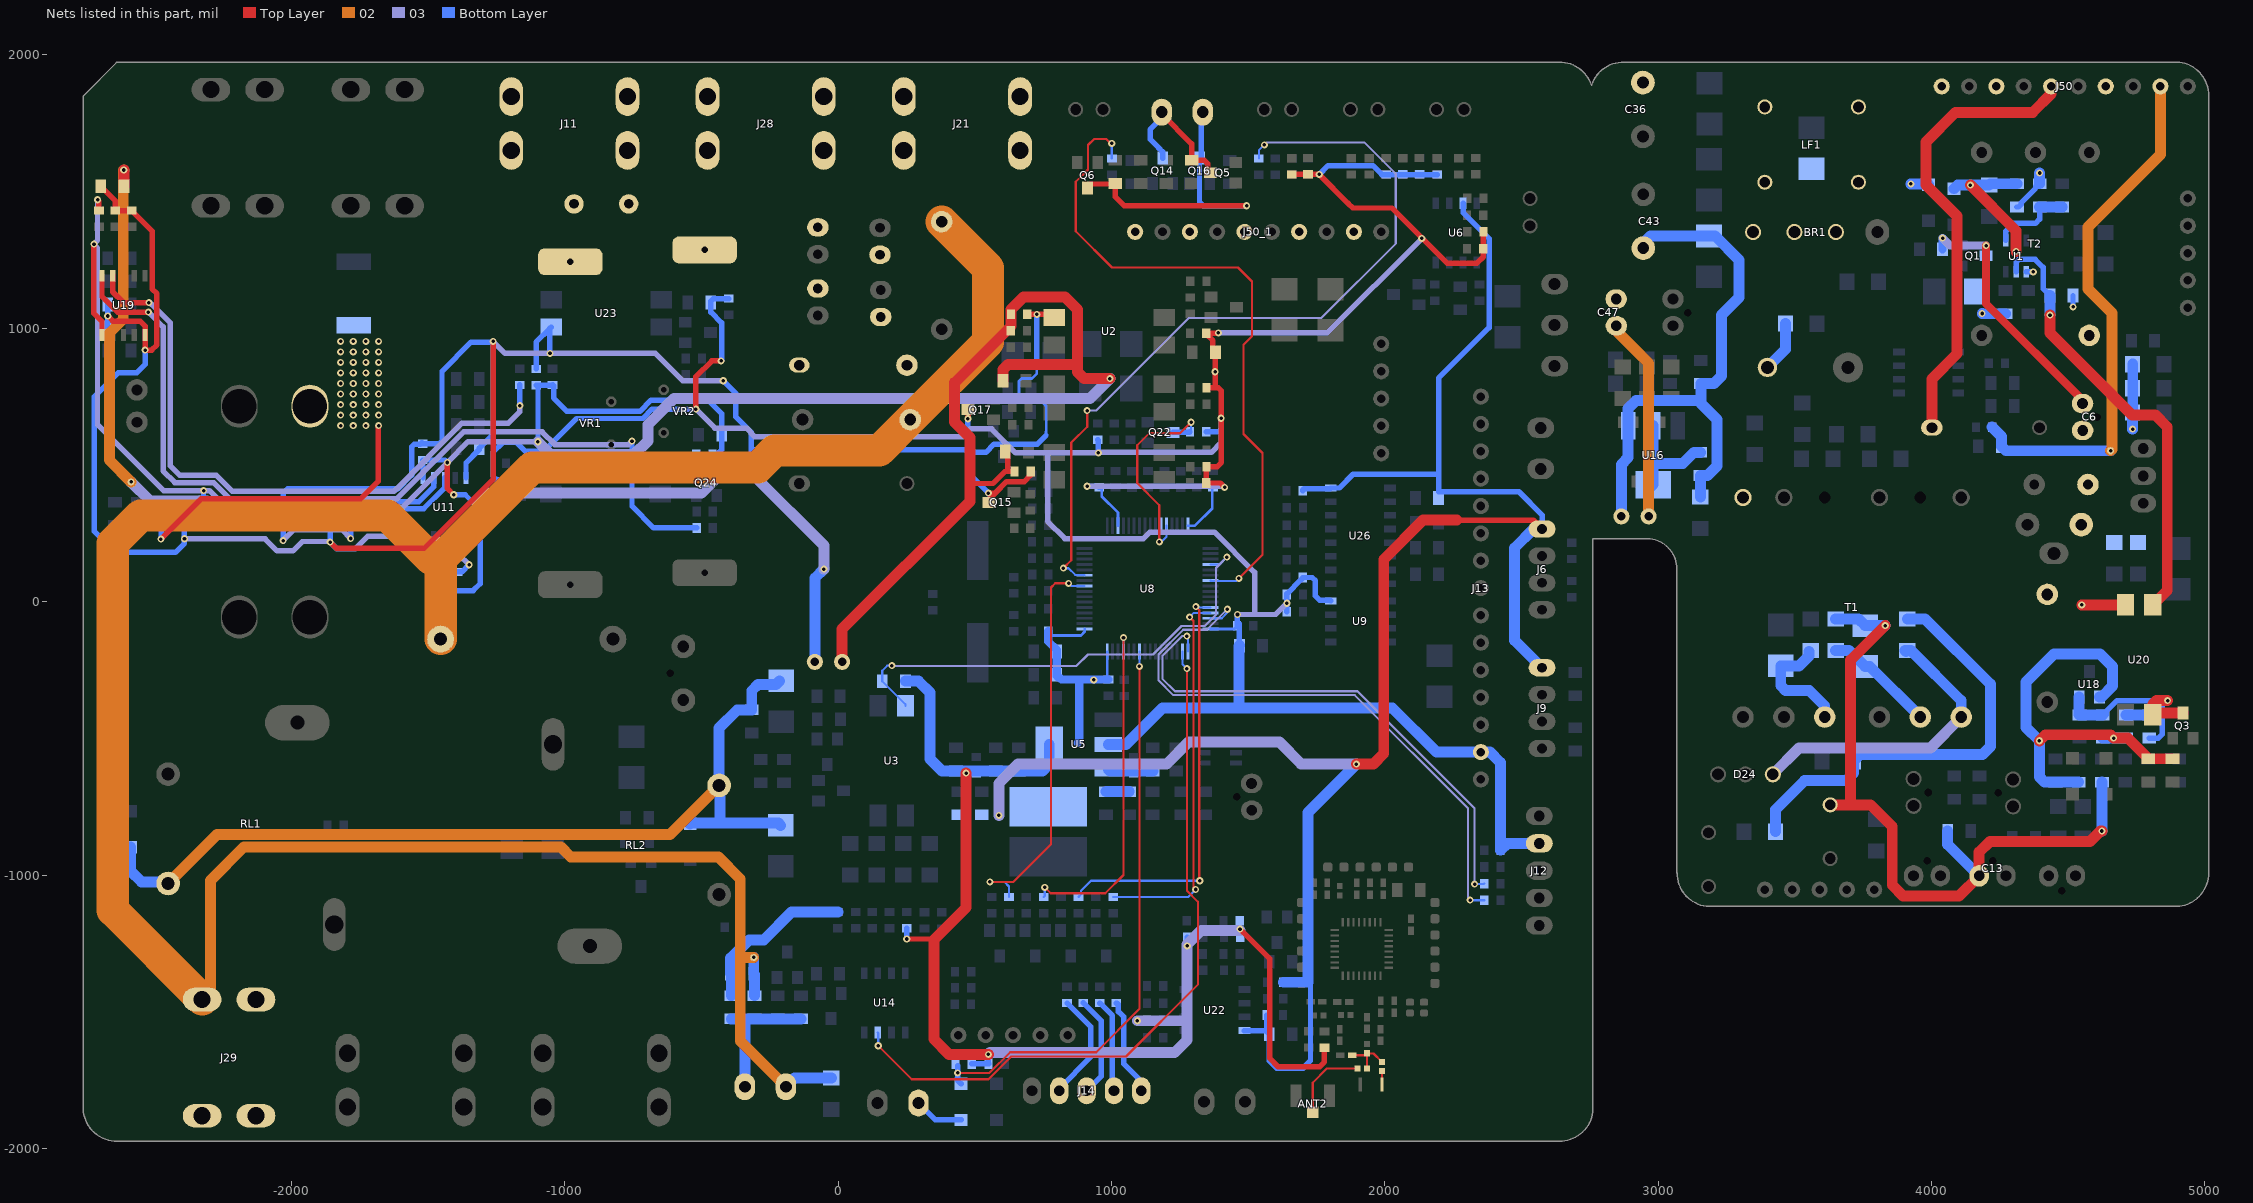
[diagram p0: the nets of this part, all layers, seen from the top]
# Altium PCB MISC105418.PcbDoc (part 4 of 7)
Units mil, origin at the board's own origin, x right, y up, seen from the top; angles counter-clockwise.
Board outline 7774.32 x 3947.04 mil, 4 copper layers (Top Layer, 02, 03, Bottom Layer), stack 30.635 mil thick; 459 components, 285 nets, 1258 pads, 468 vias.
Unrouted connection lines stored in the file: 23.

## Via types
v1: diameter 26, hole 13, Top Layer to Bottom Layer, tented both sides, 468 vias

## Nets (pads, with @x,y where several pads share a name; then routed paths per layer and width w, separated by ;. In a path a pad name is that pad's centre, name@x,y a point inside that pad or via, vN(x,y) a via of type N, cw(c..) or ccw(c..) an arc to the next point about the centre after c; other vN are vias at no path point) (continued)
CHECK-CP: R60.2 R100.2 R103.1 | length 600.5
  Bottom Layer w40: R100.2@-390.91,-1441.5 -390.91,-1363.14 R103.1@-393.23,-1360.82 -392.91,-1360.5 -392.91,-1303.91 -326,-1237 -272,-1237 -169.98,-1134.98 R60.2@-1.11,-1134.98
COIL: C45.1 D12.2 D13.2 D14.2 D15.2 RL1.3 RL2.3 | length 3423.4
  02 w40: RL1.3@-2450.87,-1031 -2271.87,-852 -615.27,-852 RL2.3@-435.21,-671.94
  Bottom Layer w40: D12.2@-2588,-897.94 -2588,-985.39 -2548.57,-1024.82 -2457.06,-1024.82 RL1.3@-2450.87,-1031 ; D13.2@-541.68,-812.74 -539,-810.06 -433.69,-810.06 ; RL2.3@-435.21,-671.94 -435.21,-462.21 -369.05,-396.05 -316.32,-396.05 C45.1@-316,-395.73 -316,-326 -292.57,-302.57 -226.51,-302.57 D14.2@-213.81,-289.87 ; RL2.3@-432.71,-674.45 -432.71,-809.07 -433.69,-810.06 ; D15.2@-210,-818.2 -218.14,-810.06 -433.69,-810.06
CP: C51.1 J26.2 R97.2 R99.1 R100.1 | length 504.5
  Bottom Layer w40: R100.1@-390.91,-1526.14 -338.14,-1526.14 ; J26.2@-341.02,-1774.5 -341.02,-1529.02 -338.14,-1526.14 ; R97.2@-135.91,-1526.14 R99.1@-220.91,-1526.14 C51.1@-305.91,-1526.14 -338.14,-1526.14
CP-ADC-PB1: U8.27
CP-PWM-PA15: U8.50 U14.3 | length 2653.9
  Top Layer w8: v1(147,-1624.43) 269.57,-1747 550,-1747 633,-1664 1053,-1664 1316,-1401 1316,-1098.05 1276,-1058.05 v1(1276,-245)
  Bottom Layer w8: U14.3@145.09,-1575.76 147,-1577.67 v1(147,-1624.43) ; U8.50@1260.05,-182.81 1260.05,-229.05 v1(1276,-245)
D3.3V: C29.1 C31.1 C32.1 C41.2 C54.1 C67.2 C68.2 C69.2 C72.2 C91.2 C95.1 C97.2 C103.1 C104.1 C105.1 C106.1 C107.1 C108.1 C109.2 C115.2 C118.2 FB2.1 J12.4 J13.14 L31.1 R41.1 R53.1 R54.1 R55.1 R63.2 R82.1 R86.2 R107.2 R115.2 R118.2 R133.2 R150.2 R152.2 R154.2 R157.2 R163.2 R173.1 R196.2 R197.1 R233.1 R237.1 R240.1 U5.2 U8.1 U8.19 U8.32 U8.48 U8.64 U9.8 | length 17731.5
  Top Layer w20: v1(-520,704) -520,823 -462,881 v1(-428,881) ; v1(251,-1234) 350,-1234 ; R163.2@1347.83,781.91 1391.09,781.91 1402,771 1402,509 1386.41,493.41 R86.2@1347.83,493.41 1347.24,492.82 1347.24,434.59 C91.2@1346.65,434 1398,434 v1(1414,418) ; 1379.32,781.91 1380.37,782.96 R63.2@1380.37,911.91 1370.69,921.59 1370.69,955.31 1346.65,979.35 C54.1@1346.65,981.91 1389.91,981.91 v1(1391,983) ; v1(1470,-1198) 1579,-1307 1579,-1671 1610,-1702 1761,-1702 1779.09,-1683.91 FB2.1@1779.09,-1632.22 ; R157.2@1659.85,1562.24 1660.23,1562.62 1759.62,1562.62 v1(1760,1563) 1865.88,1457.12 1865.88,1457 1882.88,1440 2026,1440 2228,1238 2337,1238 2359.91,1260.91 C118.2@2359.91,1290.95 2359.91,1352.24 R152.2@2361.09,1353.42
  Top Layer w40: v1(468.5,-627) 468.5,-1119.5 350,-1238 350,-1600 406,-1656 v1(550,-1656)
  03 w20: v1(-520,704) -451,635 -336,635 -305,604 455.63,604 483.63,632 561.56,632 649.56,544 766,544 ; v1(911,422) 1410,422 v1(1414,418) ; v1(1391,983) 1789,983 v1(2135,1329) ; v1(1401,671) 1401,582 1365,546 954,546 v1(952,544) 766,544 ; v1(1461,-47) 1525,-47 ; v1(1641.37,-5.75) 1600.12,-47 1525,-47 ; 766,544 766,293.81 829.24,230.57 1116.57,230.57 1140,254 1376.72,254 1523.36,107.36 1523.36,-45.36 1525,-47
  03 w40: v1(550,-1656) 556,-1650 1230,-1650 1277,-1603 1277,-1534 ; v1(1095,-1533) 1276,-1533 1277,-1534 ; v1@1470,-1203 1328,-1203 1277,-1254 v1(1277,-1259) 1277,-1534
  Bottom Layer w10: C109.2@776.89,-100.13 C109.2@768.53,-108.5 768.53,-121.53 771,-124 888,-124 901.78,-110.22 U8.1@901.78,-100.13 ; C105.1@955,418.28 964.02,409.25 964.02,385.68 1023.83,325.87 U8.19@1023.83,277.82 ; U8.64@984.46,-182.81 984.46,-280.01 C104.1@989,-284.55 ; U8.32@1279.73,277.82 1304.82,277.82 1368.44,341.44 1368.44,418.28 C103.1@1371,418.28 1413.72,418.28 v1(1414,418) ; U8.48@1362.41,-100.13 1449.12,-100.13 C106.1@1467.8,-81.45
  Bottom Layer w19.68: v1(1095,-1533) 1095.35,-1532.65 1129.18,-1532.65 R173.1@1129.53,-1532.29
  Bottom Layer w20: C97.2@-1216.43,386.5 -1215.25,387.69 R133.2@-1215.25,446.23 -1250.28,446.23 -1262,457.94 -1262,547 -1226,583 -1177,583 -1145,551 -1076,551 -957,670 -714,670 -680,704 v1@-521.62,704 ; v1(-428,881) -426,883 -426,1019.77 -465.58,1059.36 R107.2@-465.58,1094.5 -465.58,1099.04 -455.9,1108.72 C95.1@-400,1108.72 ; v1(251,-1234) 251,-1194.87 R82.1@251.44,-1194.43 ; R55.1@489.15,-1690.94 R240.1@550.25,-1690.94 550,-1690.69 v1(550,-1656) ; v1(911,422) 951.28,422 C105.1@955,418.28 ; R41.1@950.04,592.28 952,590.32 v1(952,544) ; v1@1276.63,-1259 R115.2@1276.63,-1227.17 ; R237.1@1346.45,621 1393,621 1401,629 v1(1401,671) ; C106.1@1459.28,-89.98 C106.1@1459.28,-88 1459.28,-48.72 v1(1461,-47) ; C107.1@1467.8,-161 C106.1@1467.8,-81.45 ; R53.1@1641.37,-37.5 v1(1641.37,-5.75) R54.1@1641.37,25.99 1641.37,28.55 1693.4,80.57 1694.48,80.57 1699.64,85.73 C41.2@1699.64,88.29 1734.28,88.29 1746,76.57 1746,21 1762.21,4.79 1799.62,4.79 U9.8@1801.83,2.58 ; v1(1760,1563) 1792,1595 1956,1595 1988.72,1562.28 R154.2@2004.81,1562.28 R150.2@2191.62,1562.28
  Bottom Layer w30: C109.2@768.53,-108.5 768.68,-108.65 768.68,-145.87 C108.1@800,-177.18 ; C108.1@800,-187.28 R197.1@800,-267 800,-272.31 804.68,-277 810,-277 817.55,-284.55 882,-284.55 ; 876,-517 882,-511 882,-284.55 ; C104.1@989,-284.55 882,-284.55
  Bottom Layer w40: R196.2@246.32,-291 294,-291 336,-333 336,-575 380.29,-619.29 L31.1@431.09,-619.29 C31.1@576.09,-619.29 C29.1@661.09,-619.29 747.71,-619.29 772.35,-594.65 U5.2@772.35,-522.5 ; U5.2@988.09,-522.5 1052.5,-522.5 1186,-389 1467,-389 ; C107.1@1467.8,-161 1467,-161.8 1467,-389 ; J12.4@2565.09,-884.3 2448.29,-884.3 R233.1@2423.09,-909.5 2423.09,-589.09 2384.3,-550.3 J13.14@2351.09,-550.3 2188.3,-550.3 2027,-389 1467,-389
  other v1: 935,-286 1379,841
D5V: C17.1 C20.1 C21.1 C22.1 C25.1 C26.1 C28.1 C30.1 C33.1 J6.1 J9.1 L29.2 R36.1 R178.1 U5.3 U6.3 U22.8 U26.16 | length 7729.1
  Top Layer w20: 2263,298 2542.8,298 J6.1@2575.09,265.7
  Top Layer w40: v1(1896,-594) 1958,-594 1996,-556 1996,154.31 2139.69,298 2263,298
  03 w40: v1(588,-782) 588,-664.5 658.5,-594 1202,-594 1282,-514 1614,-514 1694,-594 v1(1896,-594)
  Bottom Layer w20: U22.8@1486.06,-1568.96 1563.48,-1568.96 C21.1@1568.13,-1573.61 ; C22.1@1568.13,-1512.14 C21.1@1568.13,-1573.61 ; C20.1@1699.64,405.7 1699.64,408.26 1704.8,413.42 1799.54,413.42 U26.16@1801.83,415.7 1833.7,415.7 1884,466 2194,466 ; 1728,-1355 1728,-1679 1701,-1706 1604,-1706 1576.65,-1678.65 C21.1@1576.65,-1582.14 C21.1@1568.13,-1573.61 ; U6.3@2286.09,1457.5 2286.09,1422.91 2381,1328 2381,1002.27 2196.32,817.59 2196.32,402 2490,402 2575.09,316.91 J6.1@2575.09,265.7 J6.1@2543.7,265.7
  Bottom Layer w40: C33.1@980.08,-695.17 R36.1@1065.08,-695.17 ; U5.3@988.09,-613.44 993.94,-619.29 C25.1@1151.09,-619.29 ; R178.1@1628.76,-1392.14 1719,-1392.14 1719,-771 v1(1896,-594) ; J6.1@2543.7,265.7 2475,197 2475,-141.57 J9.1@2575.09,-241.66
DB-RX7: R112.2 U19.10 | length 3264.1
  Top Layer w20: U19.10@-2692.74,1192.27 -2692.74,1115.74 -2636,1059 v1(-2523,1059)
  03 w20: v1(-2523,1059) -2469,1005 -2469,478 -2426.23,435.23 -2284.56,435.23 -2225.33,376 -1615.23,376 -1407.23,584 -1370.23,621 -1083.09,621 -1036.09,574 -767,574 v1(-754,587)
  Bottom Layer w20: v1(-754,587) -754,349 -674.5,269.5 R112.2@-517.57,269.5
DB-TX7: R105.2 U19.9 | length 2376.1
  Top Layer w20: U19.9@-2653.37,1192.27 -2653.37,1133.37 -2614,1094 v1(-2521,1094)
  03 w20: v1(-2521,1094) -2519.38,1094 -2513.38,1088 -2510.99,1088 -2443,1020.01 -2443,497 -2408,462 -2274.56,462 -2215.56,403 -1625,403 -1375,653 -1206,653 -1164,695 v1(-1164,717)
  Bottom Layer w20: R105.2@-1164.5,792.75 -1164.25,792.5 -1164.25,717.25 v1(-1164,717)
DBGND: C50.1 C64.2 C74.1 C76.1 C90.1 C92.2 C93.1 C96.1 C98.2 C99.1 C100.2 Q15.3 Q17.3 Q24.3 R96.2 R188.2 R189.1 R190.1 R232.2 R264.1 U2.3 U11.5 U19.5 U23.3 | length 10982.3
  Top Layer w20: R96.2@-2696.85,1519 -2644,1466.15 R190.1@-2644,1430.49 R189.1@-2584,1430.49 -2509,1355.49 -2509,1144 -2492,1127 -2492,939 -2511,920 v1(-2535,920) -2535.13,920.13 -2535.13,975.6 U19.5@-2535.26,975.73 -2535.26,1007.83 -2553.43,1026 -2652.62,1026 v1(-2671.55,1044.93) ; v1(-1858,218) -1836,196 -1513,196 -1262,447 v1(-1262,952) ; v1(475,669) 475.48,669.48 Q17.3@475.48,702.6 ; v1(550,397) 550.22,397.22 574.78,397.22 ; Q15.3@551.37,363 551.37,373.82 574.78,397.22 ; C50.1@692.07,1050.81 v1(727,1050.81) 779.31,1050.81 U2.3@791.21,1038.91 ; C90.1@704.52,476 704.52,462.52 681,439 616.56,439 574.78,397.22
  03 w20: v1(-2391,230) -2096,230 -2052,186 -1994,186 -1960,220 -1860,220 v1(-1858,218) -1834.31,194.31 -1766,194.31 -1721.31,239 -1587,239 -1519,171 -1386,171 v1(-1350,135) ; v1(-1262,952) -1218,908 v1(-1054,908) -668,908 -568,808 v1(-420,808)
  Bottom Layer w10: 727,872 727,834 709,816 671,816 662,807 662,748 675,735 742.56,735 761,716.56 761,622.06 760.49,621.55 760.49,608
  Bottom Layer w20: C100.2@-2671.55,1002.7 v1(-2671.55,1044.93) R188.2@-2671.55,1087.17 ; C99.1@-2561.45,278.77 C99.1@-2560.91,279.31 -2521.22,319 -2431.86,319 C98.2@-2392.18,279.31 ; v1(-2535,920) -2535,868 -2565,838 -2633,838 -2721,750 -2721,257 -2644,180 -2424,180 -2391,213 v1(-2391,230) -2391.59,230.59 -2391.59,278.72 C98.2@-2392.18,279.31 ; C92.2@-2321.4,313.04 -2323.96,313.04 -2348,289 -2382.49,289 C98.2@-2392.18,279.31 ; C76.1@-2030.15,363.96 -2030.15,395.85 -2013,413 -1610,413 -1560,463 -1560,566.33 -1550.33,576 -1528.72,576 -1523,581.72 C64.2@-1519,577.72 -1458.28,577.72 -1449,587 -1449,842.5 -1342.5,949 -1265,949 v1(-1262,952) -1262,611.98 R232.2@-1312.47,561.5 ; C74.1@-1861.91,279.31 -1858,275.41 v1(-1858,218) ; R264.1@-1391.91,108.78 -1376.22,108.78 v1(-1350,135) ; U11.5@-1361.17,452.77 -1361.17,507.5 R232.2@-1312.74,555.93 ; C93.1@-1104.5,851.02 -1104.5,949.31 U23.3@-1054,999.81 ; v1(-1054,908) U23.3@-1054,999.81 ; U23.3@-1049.31,1004.5 U23.3@-1054,999.81 ; C96.1@-518.75,539.5 -518.75,496.75 -502.76,480.76 Q24.3@-481.68,480.76 -339.24,480.76 -317,503 -317,556 ; v1(-420,808) -375,763 -375,677 -317,619 -317,556 ; 475,547 v1(475,669) ; 475,556 -317,556 ; v1(550,397) 475,472 475,546 541,546 571,576 728.49,576 760.49,608 ; 727,872 v1(727,1050.81) ; R232.2@-1312.74,555.93 -1312.47,556.19 R232.2@-1312.47,561.5 ; R232.2@-1312.74,555.93 -1312.74,561.24 R232.2@-1312.47,561.5
EARTH: C51.2 C120.1 FB1.2 J21.1 J26.1 J29.1 J50.9 J50_1.9 R103.2 R192.1 Y2.2 Y3.1 ZC1.1 | length 11901
  02 w40: J29.1@-2326.43,-1455.4 -2296,-1424.98 -2296,-1020 -2174,-898 -1014,-898 -978,-934 -438,-934 -358,-1014 -358,-1301.42 ; v1(-308.58,-1301.42) -358,-1301.42 ; J26.1@-191.02,-1774.5 -358,-1607.52 -358,-1301.42 ; v1(4655,552) 4660,557 4660,1056 4571.94,1144.06 4571.94,1369.94 4837,1635 J50.9@4837,1885
  02 w118.11: J29.1@-2326.43,-1455.4 -2653,-1128.83 -2653,214 -2552,315 -1648,315 -1489.04,156.04 -1453.96,156.04 ; ZC1.1@-1453.96,-137 -1453.96,156.04 ; Y2.2@379,1389.85 548,1220.85 548,950.15 Y3.1@263.85,666 150.85,553 -232,553 -294,491 -1119,491 -1453.96,156.04
  Bottom Layer w40: v1(-308.58,-1301.42) R103.2@-308.58,-1360.82 -305.91,-1363.5 C51.2@-305.91,-1441.5 ; J26.1@-191.02,-1774.5 -159.46,-1742.94 FB1.2@-24.91,-1742.94 ; C120.1@4221.5,638.5 4255.22,604.78 R192.1@4255.22,568.5 4271.72,552 v1(4655,552)
EL3.3V: 2*2.54.1 ?.1 C47.1 C49.2 C50.2 C64.1 C90.2 C92.1 C93.2 C96.2 R61.2 R66.1 R89.1 R104.2 R110.1 R147.2 R162.2 U11.1 U16.2 U19.1 | length 11471.1
  Top Layer w19.68: v1(-2722,1308) -2723,1307 -2723,1055.59 -2692.74,1025.33 U19.1@-2692.74,975.73 ; v1(-2709,1470) -2704,1465 R147.2@-2704,1430.49 ; v1(-1429.38,509) -1429.38,414.38 v1(-1406,391) ; 495,432 566,432 610,476 C90.2@645.07,476 ; R66.1@611.35,549 620.53,539.82 620.53,483.87
  Top Layer w40: 2*2.54.1@14.72,-220.24 14.72,-100.28 482,367 482,601 425.86,657.14 425.86,800.86 632.62,1007.62 C50.2@632.62,1050.81 632.62,1068.93 678,1114.31 829.69,1114.31 875,1069 875,876 ; R89.1@602.74,808.3 602.74,849.74 621,868 867,868 875,876 ; v1(994,816) 899,816 875,840 875,876
  02 w40: C47.1@2828.59,1008.98 2965,872.57 ?.1@2965,312
  03 w19.68: v1(-2709,1470) -2709,1321 v1(-2722,1308) -2722,1306.31 -2709,1293.31 -2709,648 -2467.23,406.23 v1(-2321,406.23) -2300.23,406.23 -2240,346 -1592.38,346 v1(-1429.38,509) -1353.38,585 v1(-1098,585)
  03 w40: v1(-1098,585) -1051,538 -746,538 -696,588 -696,647 -600,743 921,743 v1(994,816)
  Bottom Layer w19.68: C92.1@-2321.4,372.48 -2321.2,372.69 -2321.2,406.03 v1(-2321,406.23) ; U11.1@-1518.65,452.77 -1518.65,517.92 C64.1@-1519,518.28 -1438.65,518.28 v1(-1429.38,509) ; R162.2@-1452.52,109.39 R162.2@-1451.91,108.78 -1451.91,62.27 -1429.64,40 -1335,40 -1309,66 -1309,336 -1364,391 v1(-1406,391) ; C93.2@-1104.5,791.57 -1103.32,791.57 -1098,786.26 v1(-1098,585)
  Bottom Layer w20: C93.2@-1103.32,791.57 -1045.69,791.57 R104.2@-1044.5,792.75 -1040.98,789.23 -1040.98,744.98 -992,696 -724.77,696 -683.77,737 -476,737 -425.58,686.58 R110.1@-425.58,610.76 -425.58,556.42 -442.5,539.5 C96.2@-459.3,539.5
  Bottom Layer w40: ?.1@2965,312 2965,412.29 U16.2@2981,428.29 2981,503 ; U16.2@2981,644.04 2981,505 3089.65,505 3130.98,546.32 C49.2@3154,546.32
Emer-DI-PB2: Q22.3 R237.2 U8.28 | length 792.7
  Top Layer w8: v1(1175,218.65) 1175,353 1094,434 1094,572.02 1137.98,616 1250.73,616 v1(1291,656.27)
  Bottom Layer w8: v1(1175,218.65) 1182.65,218.65 1200.99,236.99 U8.28@1200.99,277.82 ; R237.2@1287,621 1291,625 v1(1291,656.27)
  Bottom Layer w20: Q22.3@1225.26,619 1285,619 R237.2@1287,621
GND: BR1.4 C1.2 C2.2 C3.2 C5.2 C6.2 C62.2 CY1.2 R7.2 R13.2 R16.2 R241.2 T1.6 U1.1 U20.4 ZD1.1 | length 969.4
  Top Layer w39.37: v1(4549,-12) 4708.8,-12 U20.4@4709.09,-11.71
  Bottom Layer w19.68: C3.2@4312.09,1443.7 4317.41,1443.7 4327.25,1453.54 4327.25,1458.86 4379.94,1511.54 4379.94,1518.5 4389.78,1528.35 C2.2@4395,1528.35 ; U1.1@4346.4,1206.52 v1(4371.61,1206.52) ; v1(4517.32,1078) C1.2@4517.32,1120
  Bottom Layer w39.37: C62.2@3399.36,857 3465.44,923.08 C5.2@3465.44,1017 ; v1(3924,1528) 3986.49,1528 ZD1.1@3989.09,1525.39 ; v1(4185,1054) 4185.84,1053.16 R7.2@4270.09,1053.16 ; C2.2@4395,1528.35 v1(4395,1568) ; v1(4735,631) 4735,691.56 R241.2@4735.44,692 R13.2@4735.44,780.5 R16.2@4735.44,869
IN: C76.2 R145.1 U11.3 | length 928.3
  03 w20: v1(-2030,223) -1989.91,263.09 -1815.09,263.09 v1(-1783,231)
  Bottom Layer w19.68: v1(-1783,231) -1783,305.67 -1780.33,308.33 -1783,311 -1754.16,339.84 -1516.16,339.84 -1439.91,416.09 U11.3@-1439.91,452.77
  Bottom Layer w20: R145.1@-2119.69,279.31 C76.2@-2030.15,279.31 -2030.15,223.15 v1(-2030,223)
IP: C74.2 R123.1 U11.2 | length 523
  Bottom Layer w20: R123.1@-1946.14,363.96 C74.2@-1861.92,364.96 ; C74.2@-1861.91,363.96 -1860.18,365.69 -1533.32,365.69 -1479.28,419.72 U11.2@-1479.28,452.77
IP2: pad.1@-1932,715 R182.1 R183.2 | length 1136.7
  Top Layer w20: v1(-2477,229) -2329,377 -1746,377 -1682.15,440.85 -1682.15,642.85 v1(-1681,644)
  Bottom Layer w20: v1(-2477,229) -2476.66,229.34 R182.1@-2476.66,279.31
  other v1: -1820,644 -1773.67,644 -1727.33,644 -1820,682.5 -1773.67,682.5 -1727.33,682.5 -1681,682.5 -1820,721 -1773.67,721 -1727.33,721 -1681,721 -1820,759.5 -1773.67,759.5 -1727.33,759.5 -1681,759.5 -1820,798 -1773.67,798 -1727.33,798 -1681,798 -1820,836.5 -1773.67,836.5 -1727.33,836.5 -1681,836.5 -1820,875 -1773.67,875 -1727.33,875 -1681,875 -1820,913.5 -1773.67,913.5 -1727.33,913.5 -1681,913.5 -1820,952 -1773.67,952 -1727.33,952 -1681,952
JTAG_TCK: R235.2 U8.49 | length 1913.2
  03 w8: v1(1276,-126) 1258.8,-126 1186.13,-198.67 1186.13,-282.13 1232,-328 1900,-328 2328,-756 v1(2328,-1033)
  Bottom Layer w8: v1(1276,-126) 1279.73,-129.73 U8.49@1279.73,-182.81 ; v1(2328,-1033) 2362.14,-1033 R235.2@2363.65,-1031.5
JTAG_TMS: R234.2 U8.46 | length 2214.6
  03 w8: v1(1424,-28) 1349,-103 1262,-103 1172,-193 1172,-288 1226,-342 1890,-342 2304,-756 2304,-1084 v1(2312,-1092)
  Bottom Layer w8: U8.46@1362.41,-60.76 1403.24,-60.76 1424,-40 v1(1424,-28) ; v1(2312,-1092) 2312.5,-1092.5 R234.2@2363.65,-1092.5
L1: BR1.3 D11.1 LF1.1
L2: F1.1 J11.1
L-3: CX2.1 J50.1 J50_1.1 L27.2 LF1.2
L-PLC: CX3.2 F1.2 J50.5 J50_1.5 L26.1 VR1.2 | length 1687.9
  Top Layer w40: CX3.2@4001.09,636.5 4001.09,815.09 4093,907 4093,1411 3980,1524 3980,1682 4088,1790 4370,1790 4437,1857 J50.5@4437,1885
LED-4: J14.5 R126.1 | length 360.6
  Bottom Layer w20: R126.1@1017.25,-1468.34 1019.81,-1468.34 1024.97,-1473.5 1024.97,-1499.29 1044,-1518.32 1044,-1690 1108.98,-1754.98 J14.5@1108.98,-1789.5
LED-Breath: J14.4 R214.1 | length 342.6
  Bottom Layer w20: R214.1@957.25,-1468.34 1003,-1514.09 1003,-1757.05 1008.98,-1763.02 J14.4@1008.98,-1789.5
LED-Breath2-PA12: R127.2 U8.45 | length 1401.9
  Top Layer w8: v1(1286,-56.68) 1300,-70.68 1300,-1045 v1(1308,-1053)
  Bottom Layer w8: R127.2@1005.98,-1080.05 1280.95,-1080.05 v1(1308,-1053) ; v1(1286,-56.68) 1286,-56.08 1301,-41.08 U8.45@1362.41,-41.08
LED-Breath-PA11: R48.2 U8.44 | length 1539.8
  Top Layer w8: v1(1309,-18.08) 1309,-19.39 1321.07,-31.46 1321.07,-528.91 1321,-528.98 1321,-1019.15 v1(1323,-1021.15)
  Bottom Layer w8: R48.2@879.04,-1080.05 888.42,-1070.66 888.42,-1057.58 925,-1021 1322.85,-1021 v1(1323,-1021.15) ; v1(1309,-18.08) 1312.32,-21.39 U8.44@1362.41,-21.39
LED-EREE: J14.3 R213.1 | length 370.2
  Bottom Layer w20: R213.1@897.25,-1468.07 962,-1532.82 962,-1736.47 J14.3@908.98,-1789.5
LED-EREE-PB8: R47.2 U8.61 | length 1281.2
  Top Layer w8: v1(756,-1045) 778,-1067 977,-1067 1044,-1000 v1(1044,-131.69)
  Bottom Layer w8: R47.2@752.1,-1080.05 756,-1076.15 v1(756,-1045) ; U8.61@1043.51,-182.81 1043.76,-182.57 1043.76,-131.93 v1(1044,-131.69)
LED-RUN: J14.2 R125.1 | length 404.6
  Bottom Layer w20: J14.2@808.98,-1789.5 808.98,-1780.02 924,-1665 924,-1554.89 R125.1@837.45,-1468.34
LED-RUN-PC1: R51.2 U8.9 | length 1468.6
  Top Layer w8: v1(555,-1025) 641.52,-1025 779,-887.52 779,52 794,67 v1(843,67)
  Bottom Layer w8: v1(555,-1025) 608,-1025 625.16,-1042.16 R51.2@625.16,-1080.05 ; v1(843,67) 852.65,57.35 U8.9@901.78,57.35
M+: J15.1 Q5.3 Q14.3 R136.1 | length 528.2
  Top Layer w20: J15.1@1184.09,1790.5 1184.09,1783.91 1293.26,1674.74 R136.1@1293.26,1614.34 1339.66,1614.34 1351.37,1602.63 1351.37,1578.69 1361.06,1569 Q5.3@1362,1569
  Bottom Layer w20: J15.1@1184.09,1790.5 1184.09,1769.56 1141,1726.47 1141,1692 1173,1660 1173,1658.99 1187.09,1644.89 Q14.3@1187.09,1622.14
M-: J15.2 Q6.3 Q16.3 R130.1 | length 1164.3
  Top Layer w19.68: Q6.3@912.26,1513.82 912.26,1517.76 922.1,1527.6 1012.18,1527.6 R130.1@1014.26,1529.68 1014.26,1480.74 1047,1448 v1(1494,1448)
  Bottom Layer w19.68: Q16.3@1322.09,1622.14 1322.09,1461.91 1336,1448 v1(1494,1448)
  Bottom Layer w20: Q16.3@1322.09,1622.14 1328.09,1628.14 1328.09,1784.5 J15.2@1334.09,1790.5
M-N-DRV-PC8: R57.2 U8.39 | length 2484.8
  Top Layer w8: v1(1001,1676) 997.64,1676 981.64,1692 935.81,1692 914,1670.19 914,1581 869.09,1536.09 869.09,1354.91 1001.84,1222.16 1462.84,1222.16 1514,1171 1514,971 1483,940 1483,613 1552.44,543.56 1552.44,171.44 v1(1466,85)
  Bottom Layer w8: v1(1001,1676) 1001,1621.78 R57.2@1002.09,1620.69 ; U8.39@1362.41,77.03 1363.72,75.72 1456.72,75.72 v1(1466,85)
M/ScR-DRV-PC3: R56.1 U8.11 | length 2928
  Top Layer w8: v1(824.18,122.82) 853,151.64 853,582 911,640 v1(911,699)
  03 w8: v1(911,699) 944.67,699 1283.67,1038 1768.4,1038 2040,1309.6 2040,1565 1926,1679 1567,1679 v1(1559,1671)
  Bottom Layer w8: v1(824.18,122.82) 824.86,122.14 842.86,122.14 867.12,97.88 900.62,97.88 U8.11@901.78,96.72 ; R56.1@1539.09,1620.69 1539.09,1651.09 v1(1559,1671)
Mecha1-DI: D17.2 J16.2 | length 181.7
  Bottom Layer w20: J16.2@293.98,-1833.94 355.98,-1895.94 D17.2@449.98,-1895.94
Mecha1-DI-PB6: D17.1 R55.2 U8.58 | length 2140.5
  Top Layer w8: v1(437,-1724) 553.2,-1724 629.2,-1648 944,-1648 1102,-1490 v1(1102,-237)
  Bottom Layer w8: v1(1102,-237) 1102.28,-236.72 1102.28,-183.09 U8.58@1102.57,-182.81
  Bottom Layer w20: R55.2@437,-1698.24 v1(437,-1724) 437,-1751.08 D17.1@449.98,-1764.06
N: 2*2.54.2 ?.2 BR1.2 C36.2 C43.2 C44.1 C47.2 C49.1 D4.1 LF1.3 R95.2 R96.1 U16.1 | length 6702.7
  Top Layer w40: v1(-2613,1579) -2612.21,1578.21 R96.1@-2612.21,1519
  02 w40: v1(-2613,1579) -2615,1577 -2615,1033 -2666,982 -2666,518 v1(-2586,438)
  03 w40: v1(-2586,438) -2516,368 -2337.93,368 -2280.08,310.16 -1598.16,310.16 -1505.76,217.76 -1377.08,217.76 -1320.42,274.42 -1320.42,363.58 -1286.03,397.97 -499.35,397.97 -439.32,458 -305,458 -52,205 v1(-52,119)
  Bottom Layer w40: 2*2.54.2@-85.28,-220.24 -85.28,85.72 v1(-52,119) ; ?.2@2865,312 2865,502 2890.06,527.06 U16.1@2890.06,644.04 2890.06,707.06 2918,735 3156,735 ; C43.2@2927.36,1293.18 2971.79,1337.61 D4.1@3186,1337.61 3208.39,1337.61 3296,1250 3296,1113 3232,1049 3232,826 3203.79,797.79 C44.1@3156,797.79 3156,735 ; R95.2@3154,382.08 C49.1@3154,461.68 3180.68,461.68 3215,496 3215,666 3156,725 3156,735
N2: J28.1 J50.7 J50_1.7 L28.1 T2.3 VR2.1
N-3: CX2.2 J50.3 J50_1.3 L30.2 LF1.4
N/L-Adhe-PB15: R196.1 U3.4 U8.36 | length 1767.4
  03 w8: v1(197,-234) 198,-235 233,-235 233.39,-235 872,-235 913.8,-193.2 1152,-193.2 1256.2,-89 1341,-89 1382,-48 1382,123 v1(1422,163)
  Bottom Layer w8: v1(197,-234) 180,-234 161.68,-252.32 R196.1@161.68,-291 246.09,-375.42 U3.4@246.09,-380.71 ; U8.36@1362.41,136.09 1395.09,136.09 v1(1422,163)
NetANT1_1: ANT1.1 R260.1 | length 55.9
  Top Layer w8: ANT1.1@1989.09,-1773.5 R260.1@1989.09,-1717.58
NetANT2_1: ANT2.1 R261.2 | length 294.1
  Top Layer w8: ANT2.1@1736,-1868.02 1736,-1760 1787.97,-1708.03 R261.2@1900.51,-1708.03
NetC1_1: C1.1 U1.2 U20.3 | length 1645.1
  Top Layer w40: v1(4433,1048.29) 4433,983 4733.5,682.5 4818.5,682.5 4862,639 4862,41.2 U20.3@4809.09,-11.71
  Bottom Layer w20: U1.2@4309,1206.52 4309,1242 4319,1252 4379,1252 4408,1223 4408,1144.68 C1.1@4432.68,1120
  Bottom Layer w40: C1.1@4432.68,1120 4433,1119.68 v1(4433,1048.29)
NetC2_1: C2.1 R9.1 U1.4 | length 303.6
  Bottom Layer w19.68: U1.4@4271.6,1321.09 4271.6,1355.6 4300,1384 4380,1384 4395.09,1399.09 C2.1@4395.09,1443.7
  Bottom Layer w39.37: C2.1@4395.09,1443.7 R9.1@4478.09,1443.7
NetC3_1: C3.1 D20.2 R8.2 U1.5 | length 589.6
  Top Layer w39.37: v1(4142,1523.9) 4309,1356.9 v1(4309,1281)
  Bottom Layer w19.68: v1(4309,1281) U1.5@4309,1321.09
  Bottom Layer w39.37: D20.2@4082.09,1510.43 4095.56,1523.9 v1(4142,1523.9) R8.2@4210.09,1523.9 4214.54,1528.35 C3.1@4312.09,1528.35
NetC4_1: C4.1 L11.1 R260.2 R261.1 | length 179.6
  Top Layer w8: C4.1@1880.55,-1659.03 1928.09,-1659.03 L11.1@1934.59,-1652.54 ; R261.1@1934.59,-1708.03 L11.1@1934.59,-1652.54 ; R260.2@1989.09,-1683.5 1958.13,-1652.54 L11.1@1934.59,-1652.54
NetC6_1: C6.1 D22.2 Q1.3 R11.1 | length 1135.9
  Top Layer w30: v1(4199.35,1302.65) 4199.35,1089.65 4552.09,736.91 C6.1@4552.09,724.5
  03 w30: v1(4040.22,1329.78) 4067.35,1302.65 v1(4199.35,1302.65)
  Bottom Layer w30: R11.1@4040.22,1289.13 v1(4040.22,1329.78) ; D22.2@4199.35,1102 Q1.3@4199.35,1265.5 v1(4199.35,1302.65)
NetC7_1: C7.1 R14.2 R17.2 R19.2
NetC8_1: C8.1 D24.1 T1.12 | length 1115.5
  03 w40: D24.1@3419.09,-631.5 3515.59,-535 3995.38,-535 T1.12@4108.31,-422.07
  Bottom Layer w40: C8.1@3902.09,-178.52 C8.1@3906.55,-182.97 ; C8.1@3911,-178.52 3924.52,-178.52 4108.31,-362.31 T1.12@4108.31,-422.07
NetC8_2: C8.2 R22.1 R23.1 | length 1618.5
  Bottom Layer w40: R22.1@3428.65,-841.5 3428.65,-761.35 3535,-655 3686,-655 3713.65,-627.35 R23.1@3713.65,-584 3738.65,-559 4186,-559 4215,-530 4215,-302 3976.4,-63.4 C8.2@3911,-63.4
NetC9_1: C9.1 Q3.3 R21.2 R24.1 U18.K U20.2 | length 803.8
  Top Layer w40: v1(4863,-362) 4822,-362 4809.09,-374.91 U20.2@4809.09,-413.28 4815.14,-407.24 Q3.3@4919.09,-407.24
  Bottom Layer w20: C9.1@4626.09,-414.5 4638,-414.5 4638,-402.59 4678.59,-362 4844,-362 ; R24.1@4796.09,-499.14 4829.86,-499.14 4844,-485 4844,-362 ; v1(4863,-362) 4844,-362
  Bottom Layer w40: U18.K@4539.69,-348.76 4539.69,-413.09 R21.2@4541.09,-414.5 C9.1@4626.09,-414.5
NetC9_2: C9.2 C12.2 R26.2 R27.1 R28.2 R29.1 U18.R | length 1651.6
  Top Layer w40: v1(4394,-509) 4416,-487 4653.86,-487 v1(4666,-499.14) 4717.46,-499.14 R28.2@4793,-574.68 R26.2@4881,-574.68
  Bottom Layer w40: R27.1@4538.09,-660.5 R29.1@4453.09,-660.5 4413.5,-660.5 4394,-641 v1(4394,-509) 4345,-460 4345,-294 4448,-191 4616,-191 4662,-237 4662,-309 4622.24,-348.76 U18.R@4614.5,-348.76 ; C9.2@4626.09,-499.14 v1(4666,-499.14) C12.2@4711.09,-499.14
NetC10_1: C10.1 D25.1 T1.11 | length 410.5
  Bottom Layer w40: C10.1@3649.09,-178.52 3698.51,-178.52 D25.1@3757.09,-237.1 3773.73,-237.1 T1.11@3958.7,-422.07
NetC10_2: C10.2 C13.1 C80.2 D25.2 L25.1 R25.1 | length 2697.1
  Top Layer w40: L25.1@3629.09,-743.07 3704,-743.07 ; v1(3830.5,-87.5) 3704,-214 3704,-743.07 ; v1(4623.09,-838.91) 4618.09,-838.91 4580,-877 4213,-877 4174.08,-915.92 C13.1@4174.08,-1002.89 4099.97,-1077 3896,-1077 3856,-1037 3856,-822 3777.07,-743.07 3704,-743.07
  Bottom Layer w40: C10.2@3649.09,-63.4 3733,-63.4 D25.2@3757.09,-87.5 v1(3830.5,-87.5) ; C80.2@4058.77,-839.18 4058.77,-887.58 C13.1@4174.08,-1002.89 ; v1(4623.09,-838.91) R25.1@4623.09,-660.5
NetC11_1: C11.1 D26.2 T1.9 | length 439
  Bottom Layer w40: C11.1@3551.09,-182.52 3551.09,-198.91 3514.87,-235.13 D26.2@3448.09,-235.13 3448.09,-307.09 3465.5,-324.5 3552.5,-324.5 3609.09,-381.09 T1.9@3609.09,-422.07
NetC12_1: C12.1 R24.2 | length 85
  Bottom Layer w40: C12.1@4711.09,-414.5 R24.2@4796.09,-414.5